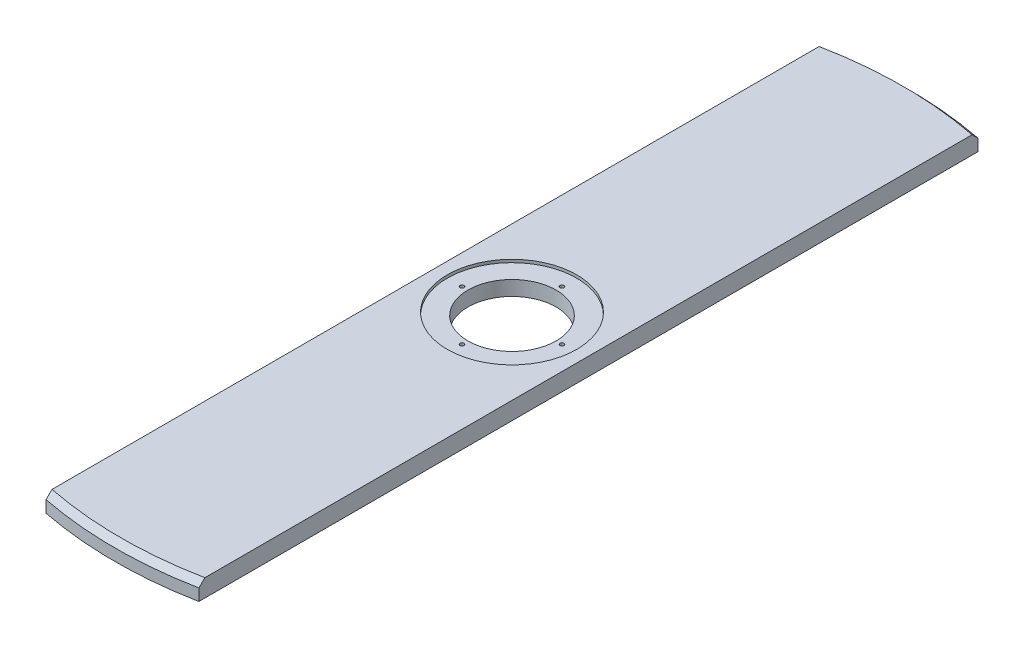
SolidWorks part; units mm, degrees
material "Q235B"
ref_plane "前视基准面" through (0, 0, 0) normal (0, 0, 1) x (1, 0, 0)
ref_plane "上视基准面" through (0, 0, 0) normal (0, 1, 0) x (1, 0, 0)
ref_plane "右视基准面" through (0, 0, 0) normal (1, 0, 0) x (0, 0, -1)
sketch "草图1" plane through (0, 0, 0) normal (0, 1, 0) x (1, 0, 0)
  circle A0 centre (0, 0) radius 810
  circle A1 centre (0, 0) radius 675 construction
  dimension "D1" = 1620
  dimension "D2" = 1350
extrude "凸台-拉伸1" add sketch "草图1" along normal blind 25
sketch "草图2" plane through (0, 25, 0) normal (0, 1, 0) x (1, 0, 0)
  circle A0 centre (0, 0) radius 730
  dimension "D2" = 1460
extrude "凸台-拉伸2" add sketch "草图2" along normal blind 5
sketch "草图3" plane through (0, 30, 0) normal (0, 1, 0) x (1, 0, 0)
  line L1 (130, -662.3632) -> (-130, -662.3632)
  line L2 (130, -662.3632) -> (130, 662.3632)
  line L3 (130, 662.3632) -> (-130, 662.3632)
  line L4 (-130, -662.3632) -> (-130, 662.3632)
  line L5 (130, -662.3632) -> (-130, 662.3632) construction
  line L6 (130, 662.3632) -> (-130, -662.3632) construction
  circle A0 centre (0, 0) radius 675
  circle A1 centre (0, 0) radius 75
  dimension "D1" = 1350
  dimension "D3" = 150
  dimension "D2" = 260
extrude "切除-拉伸1" cut sketch "草图3" against normal up to next contours L2 A0 | L4 A0 | A1
sketch "草图4" plane through (0, 30, 0) normal (0, 1, 0) x (1, 0, 0)
  circle A0 centre (0, 0) radius 110
  dimension "D1" = 220
extrude "切除-拉伸2" cut sketch "草图4" against normal blind 5
hole_wizard "M8 螺纹孔1" positions "草图5" profile "草图6" tap size "M8" standard "GB" end condition up to next
sketch "草图5" plane through (0, 25, 0) normal (0, 1, 0) x (1, 0, 0)
  line L0 (0, 0) -> (0, 85)
  circle A0 centre (0, 0) radius 85 construction
  point P0 (0, 85)
  point P15 (85, 0)
  point P16 (0, -85)
  point P17 (-85, 0)
  dimension "D1" = 170
  dimension "D2" = 4
sketch "草图6" plane through (0, 25, -85) normal (1, 0, 0) x (0, 0, 1)
  line L0 (0, 0) -> (0, 25)
  line L1 (0, 25) -> (3.4, 25)
  line L2 (3.4, 25) -> (3.4, 0)
  line L5 (3.4, 0) -> (0, 0)
  line L11 (0, -6.35) -> (0, 107.95) construction
  dimension "通孔螺纹孔钻头直径" = 6.8
  dimension "通孔螺纹孔钻头深度" = 25
cosmetic thread "孔螺蚊线1" parameters "D2"=8
cosmetic thread "孔螺蚊线2" parameters "D2"=8
cosmetic thread "孔螺蚊线3" parameters "D2"=8
cosmetic thread "孔螺蚊线4" parameters "D2"=8
hole_wizard "Ø25.5 (25.5) 直径孔1" positions "草图9" profile "草图8" hole size "Ø25.5" standard "GB" end condition up to next
sketch "草图9" plane through (0, 25, 0) normal (0, 1, 0) x (1, 0, 0)
  line L0 (0, 0) -> (0, 756.5) construction
  circle A0 centre (0, 0) radius 756.5 construction
  point P0 (-59.3543, 754.168)
  point P14 (59.3543, 754.168)
  point P15 (176.6014, 735.5978)
  point P16 (289.5, 698.9149)
  point P17 (395.2702, 645.0223)
  point P18 (491.3074, 575.2471)
  point P19 (575.2471, 491.3074)
  point P20 (645.0223, 395.2702)
  point P21 (698.9149, 289.5)
  point P22 (735.5978, 176.6014)
  point P23 (754.168, 59.3543)
  point P24 (754.168, -59.3543)
  point P25 (735.5978, -176.6014)
  point P26 (698.9149, -289.5)
  point P27 (645.0223, -395.2702)
  point P28 (575.2471, -491.3074)
  point P29 (491.3074, -575.2471)
  point P30 (395.2702, -645.0223)
  point P31 (289.5, -698.9149)
  point P32 (176.6014, -735.5978)
  point P33 (59.3543, -754.168)
  point P34 (-59.3543, -754.168)
  point P35 (-176.6014, -735.5978)
  point P36 (-289.5, -698.9149)
  point P37 (-395.2702, -645.0223)
  point P38 (-491.3074, -575.2471)
  point P39 (-575.2471, -491.3074)
  point P40 (-645.0223, -395.2702)
  point P41 (-698.9149, -289.5)
  point P42 (-735.5978, -176.6014)
  point P43 (-754.168, -59.3543)
  point P44 (-754.168, 59.3543)
  point P45 (-735.5978, 176.6014)
  point P46 (-698.9149, 289.5)
  point P47 (-645.0223, 395.2702)
  point P48 (-575.2471, 491.3074)
  point P49 (-491.3074, 575.2471)
  point P50 (-395.2702, 645.0223)
  point P51 (-289.5, 698.9149)
  point P52 (-176.6014, 735.5978)
  dimension "D1" = 1513
  dimension "D2" = 40
sketch "草图8" plane through (-59.3543, 25, -754.168) normal (1, 0, 0) x (0, 0, 1)
  line L0 (0, 0) -> (0, 25)
  line L1 (0, 25) -> (13, 25)
  line L2 (13, 25) -> (13, 0)
  line L5 (13, 0) -> (0, 0)
  line L11 (0, -6.35) -> (0, 107.95) construction
  dimension "通孔孔直径" = 26
  dimension "通孔孔深度" = 25
sketch "草图10" plane through (0, 30, 0) normal (0, 1, 0) x (1, 0, 0)
  circle A0 centre (0, 0) radius 675
extrude "切除-拉伸3" cut sketch "草图10" against normal through all both and the other way through all flip side to cut
chamfer "倒角1" distance 10 angle 45 2 edges at (0, 30, -675) (0, 30, 675)
